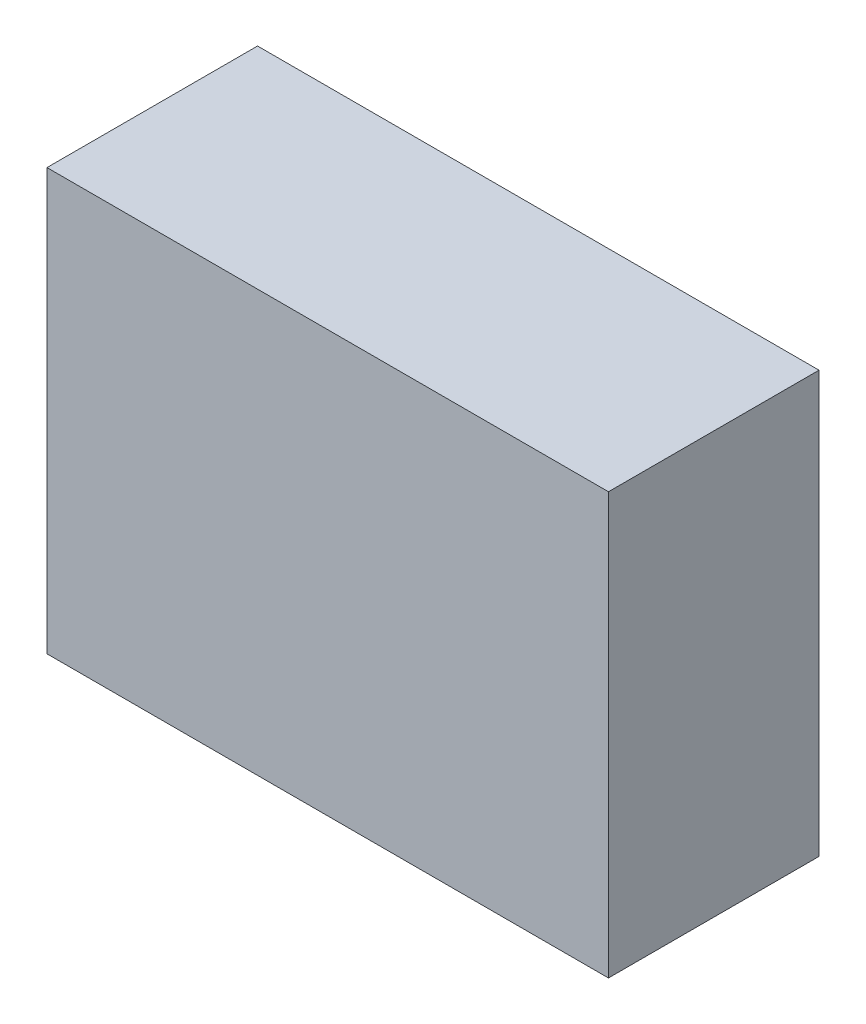
from build123d import *

# Parameters (mm, degrees)
SKETCH_1_W      = 32
SKETCH_1_H      = 24
EXTRUDE_1_DEPTH = 6


with BuildPart() as part:
    # 草图1 → 凸台-拉伸1 (new, symmetric)
    with BuildSketch(Plane.XY):
        Rectangle(SKETCH_1_W, SKETCH_1_H)
    extrude(amount=EXTRUDE_1_DEPTH, both=True)


solid = part.part
